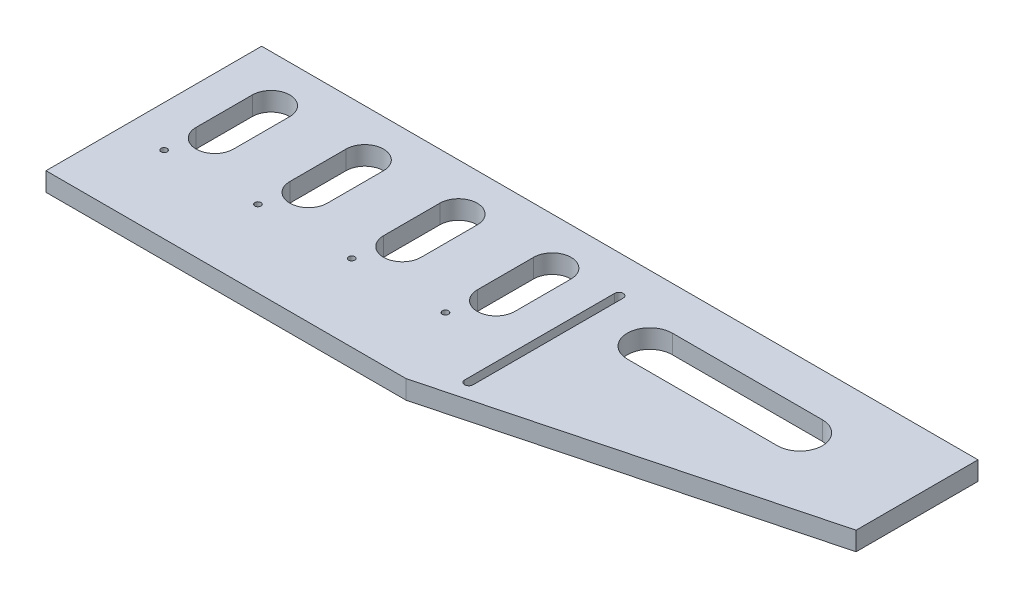
from build123d import *

# Parameters (mm, degrees)
SKETCH_1_W             = 382
SKETCH_1_H             = 80
EXTRUDE_1_DEPTH        = 10
HOLE_WIZARD_M3_1_D     = 2.5
HOLE_WIZARD_M3_1_DEPTH = 8.5
HOLE_WIZARD_M3_1_TIP   = 0.751075774
CUT_EXTRUDE_1_DEPTH    = 196.399590583
PATTERN_LINEAR_1_COUNT = 4
PATTERN_LINEAR_1_PITCH = 50
HOLE_WIZARD_M4_1_D     = 4.5
HOLE_WIZARD_M4_1_2_D   = 3.3
PATTERN_LINEAR_2_COUNT = 4
PATTERN_LINEAR_2_PITCH = 50
HOLE_WIZARD_M4_2_D     = 3.3
HOLE_WIZARD_M4_2_DEPTH = 10.1
HOLE_WIZARD_M4_2_TIP   = 0.991420021
CUT_EXTRUDE_3_DEPTH    = 10
MOVE_FACE_1_BY         = 35
CUT_EXTRUDE_4_DEPTH    = 206.440989094
CHAMFER_1_SIZE         = 190
CHAMFER_1_SIZE2        = 50
CUT_EXTRUDE_2_DEPTH    = 206.440989094


with BuildPart() as part:
    # 草图1 → 凸台-拉伸1 (new body)
    with BuildSketch(Plane(origin=(0, 0, 0), x_dir=(1, 0, 0), z_dir=(0, 1, 0))):
        Rectangle(SKETCH_1_W, SKETCH_1_H)
    extrude(amount=EXTRUDE_1_DEPTH)

    # M3 螺纹孔1
    with Locations(Plane(origin=(0, 0, -40), x_dir=(-1, 0, 0), z_dir=(0, 0, -1))):
        with Locations((187, 5), (-187, 5)):
            Hole(HOLE_WIZARD_M3_1_D / 2, depth=HOLE_WIZARD_M3_1_DEPTH)
            with Locations((0, 0, -(HOLE_WIZARD_M3_1_DEPTH + HOLE_WIZARD_M3_1_TIP / 2))):  # 118° drill point
                Cone(0, HOLE_WIZARD_M3_1_D / 2, HOLE_WIZARD_M3_1_TIP, mode=Mode.SUBTRACT)

    # 草图4 → 切除-拉伸1 (cut, through all)
    with BuildSketch(Plane(origin=(0, 10, 0), x_dir=(1, 0, 0), z_dir=(0, 1, 0))):
        with BuildLine():
            Line((-1, 15), (-1, -15))
            ThreePointArc((-1, -15), (-11, -25), (-21, -15))
            Line((-21, -15), (-21, 15))
            ThreePointArc((-21, 15), (-11, 25), (-1, 15))
        make_face()
    cut_extrude_1 = extrude(amount=-CUT_EXTRUDE_1_DEPTH, mode=Mode.SUBTRACT)

    # 阵列(线性)1: 切除-拉伸1 ×4
    with Locations(*[(-i * PATTERN_LINEAR_1_PITCH, 0, 0) for i in range(1, PATTERN_LINEAR_1_COUNT)]):
        add(cut_extrude_1, mode=Mode.SUBTRACT)

    # Hole Wizard M4 _1 (through all)
    with Locations(Plane(origin=(0, 10, 0), x_dir=(1, 0, 0), z_dir=(0, 1, 0))):
        with Locations((19.5, -11), (19.5, -31)):
            Hole(HOLE_WIZARD_M4_1_D / 2)

    # Hole Wizard M4 _1 2 (through all)
    with Locations(Plane(origin=(0, 10, 0), x_dir=(1, 0, 0), z_dir=(0, 1, 0))):
        with Locations((-19, -34)):
            hole_wizard_m4_1_2 = Hole(HOLE_WIZARD_M4_1_2_D / 2)

    # 阵列(线性)2: Hole Wizard M4 _1 2 ×4
    with Locations(*[(-i * PATTERN_LINEAR_2_PITCH, 0, 0) for i in range(1, PATTERN_LINEAR_2_COUNT)]):
        add(hole_wizard_m4_1_2, mode=Mode.SUBTRACT)

    # M4 螺纹孔2
    with Locations(Plane.ZY.offset(191)):
        with Locations((27.5, 5), (-27.5, 5)):
            Hole(HOLE_WIZARD_M4_2_D / 2, depth=HOLE_WIZARD_M4_2_DEPTH)
            with Locations((0, 0, -(HOLE_WIZARD_M4_2_DEPTH + HOLE_WIZARD_M4_2_TIP / 2))):  # 118° drill point
                Cone(0, HOLE_WIZARD_M4_2_D / 2, HOLE_WIZARD_M4_2_TIP, mode=Mode.SUBTRACT)

    # 草图14 → 切除-拉伸3 (cut)
    with BuildSketch(Plane.XZ):
        with BuildLine():
            Line((21.749999636, 33.25), (21.749999636, 28.75))
            ThreePointArc((21.749999636, 28.75), (19.499999636, 26.5), (17.249999636, 28.75))
            Line((17.249999636, 28.75), (17.249999636, 33.25))
            ThreePointArc((17.249999636, 33.25), (19.499999636, 35.5), (21.749999636, 33.25))
        make_face()
        with BuildLine():
            Line((21.749999636, 13.25), (21.749999636, 8.75))
            ThreePointArc((21.749999636, 8.75), (19.499999636, 6.5), (17.249999636, 8.75))
            Line((17.249999636, 8.75), (17.249999636, 13.25))
            ThreePointArc((17.249999636, 13.25), (19.499999636, 15.5), (21.749999636, 13.25))
        make_face()
    extrude(amount=-CUT_EXTRUDE_3_DEPTH, mode=Mode.SUBTRACT)

    # Move Face 1: a face moved outward by 35.0
    extrude(part.faces().sort_by_distance((0, 5, 40))[0], amount=MOVE_FACE_1_BY, dir=(0, 0, 1))

    # 草图15 → 切除-拉伸4 (cut, through all)
    with BuildSketch(Plane.XZ):
        with BuildLine():
            Line((21.749999636, 60), (21.749999636, -20))
            ThreePointArc((21.749999636, -20), (19.499999636, -22.25), (17.249999636, -20))
            Line((17.249999636, -20), (17.249999636, 60))
            ThreePointArc((17.249999636, 60), (19.499999636, 62.25), (21.749999636, 60))
        make_face()
    extrude(amount=-CUT_EXTRUDE_4_DEPTH, mode=Mode.SUBTRACT)

    # 倒角1
    chamfer_1_edges = [part.edges().sort_by_distance(p)[0] for p in [
        (191, 5, 75),
    ]]
    chamfer_1_side = [part.faces().sort_by_distance(p)[0] for p in [
        (0, 5, 75),
    ]]
    chamfer(chamfer_1_edges, length=CHAMFER_1_SIZE, length2=CHAMFER_1_SIZE2, reference=chamfer_1_side[0])

    # 草图5 → 切除-拉伸2 (cut, through all)
    with BuildSketch(Plane(origin=(0, 10, 0), x_dir=(1, 0, 0), z_dir=(0, 1, 0))):
        with BuildLine():
            Line((131, -7), (51, -7))
            ThreePointArc((51, -7), (39, 5), (51, 17))
            Line((51, 17), (131, 17))
            ThreePointArc((131, 17), (143, 5), (131, -7))
        make_face()
    extrude(amount=-CUT_EXTRUDE_2_DEPTH, mode=Mode.SUBTRACT)


solid = part.part
